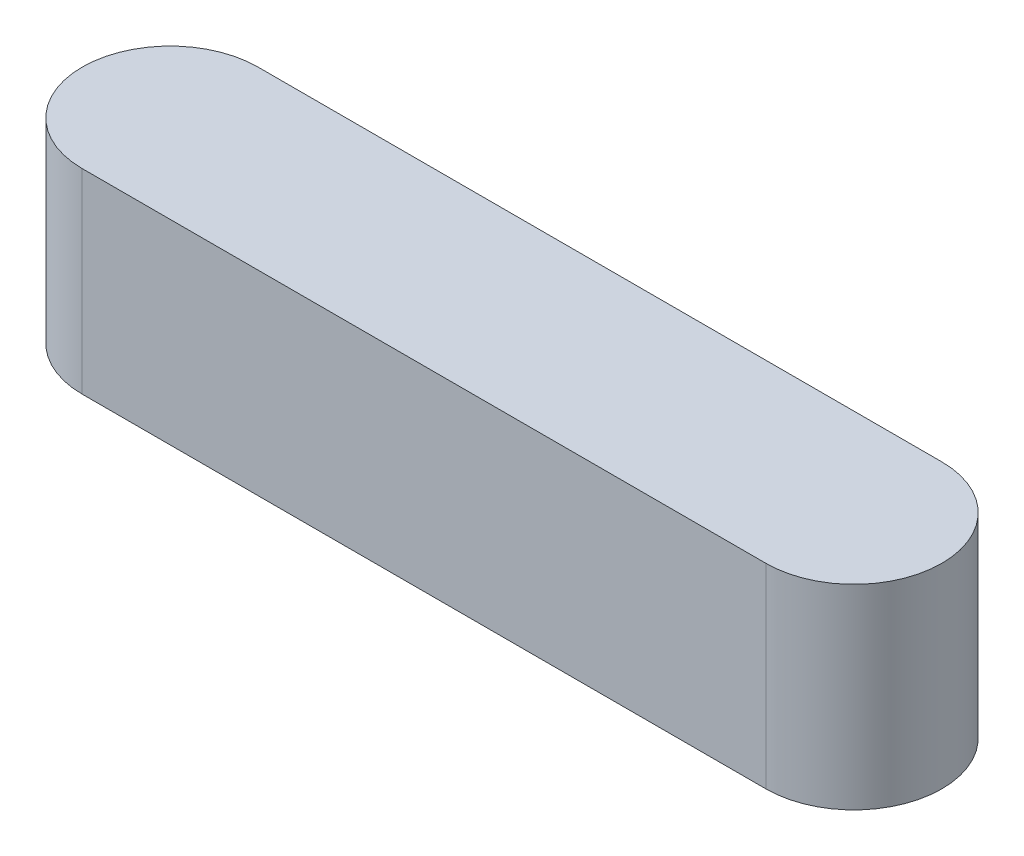
from build123d import *

# Parameters (mm, degrees)
BOSS_EXTRUDE1_DEPTH = 10
SCALE_1_SCALE       = 1.875


with BuildPart() as part:
    # Sketch1 → Boss-Extrude1 (new body)
    with BuildSketch(Plane(origin=(0, 0, 0), x_dir=(1, 0, 0), z_dir=(0, 1, 0))):
        with BuildLine():
            Line((0, 4.5), (35, 4.5))
            ThreePointArc((35, 4.5), (39.5, 0), (35, -4.5))
            Line((35, -4.5), (0, -4.5))
            ThreePointArc((0, -4.5), (-4.5, 0), (0, 4.5))
        make_face()
    extrude(amount=BOSS_EXTRUDE1_DEPTH)


with BuildPart() as part_1:
    # Scale 1: scaled about (17.5, 5, 0)
    add(part.part.scale(SCALE_1_SCALE).moved(Location((-15.3125, -4.375, 0))))


solid = part_1.part
